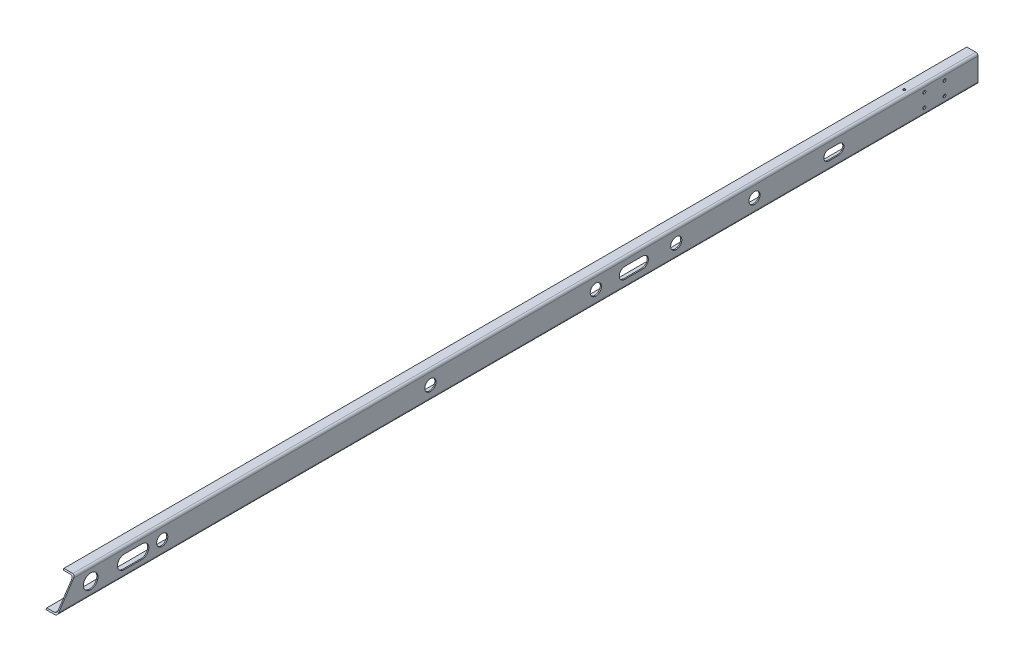
from build123d import *

# Parameters (mm, degrees)
EXTRUDE_1_DEPTH     = 4120
SKETCH_2_R          = 5
CUT_EXTRUDE_1_DEPTH = 10
SKETCH_3_R          = 6.5
SKETCH_3_R_2        = 25
SKETCH_3_R_3        = 22.5
CUT_EXTRUDE_2_DEPTH = 10
CUT_EXTRUDE_3_DEPTH = 10
SKETCH_5_R          = 6.5
CUT_EXTRUDE_4_DEPTH = 10
EXTRUDE_4_DEPTH     = 5
SKETCH_7_R          = 32.5
CUT_EXTRUDE_5_DEPTH = 10
CUT_EXTRUDE_6_DEPTH = 63


with BuildPart() as part:
    # 草图1 → 凸台-拉伸1 (new body)
    with BuildSketch(Plane.XY):
        with BuildLine():
            Line((626.175555556, -48.428888889), (666.175555556, -48.428888889))
            ThreePointArc((666.175555556, -48.428888889), (673.246623367, -45.499956701), (676.175555556, -38.428888889))
            Line((676.175555556, -38.428888889), (676.175555556, 61.571111111))
            ThreePointArc((676.175555556, 61.571111111), (673.246623367, 68.642178923), (666.175555556, 71.571111111))
            Line((666.175555556, 71.571111111), (626.175555556, 71.571111111))
            Line((626.175555556, 71.571111111), (626.175555556, 66.571111111))
            Line((626.175555556, 66.571111111), (661.175555556, 66.571111111))
            ThreePointArc((661.175555556, 66.571111111), (668.246623367, 63.642178923), (671.175555556, 56.571111111))
            Line((671.175555556, 56.571111111), (671.175555556, -33.428888889))
            ThreePointArc((671.175555556, -33.428888889), (668.246623367, -40.499956701), (661.175555556, -43.428888889))
            Line((661.175555556, -43.428888889), (626.175555556, -43.428888889))
            Line((626.175555556, -43.428888889), (626.175555556, -48.428888889))
        make_face()
    extrude(amount=EXTRUDE_1_DEPTH)

    # 草图2 → 切除-拉伸1 (cut)
    with BuildSketch(Plane(origin=(0, 71.571111111, 0), x_dir=(1, 0, 0), z_dir=(0, 1, 0))):
        with Locations(Location((651.175555556, -305, 0), (0, 0, 180))):
            Circle(SKETCH_2_R)
    extrude(amount=-CUT_EXTRUDE_1_DEPTH, mode=Mode.SUBTRACT)

    # 草图3 → 切除-拉伸2 (cut)
    with BuildSketch(Plane(origin=(676.175555556, 0, 0), x_dir=(0, 0, -1), z_dir=(1, 0, 0))):
        with Locations((-225, 41.571111111)):
            Circle(SKETCH_3_R)
        with Locations((-135, 41.571111111)):
            Circle(SKETCH_3_R)
        with Locations((-135, -18.428888889)):
            Circle(SKETCH_3_R)
        with Locations((-225, -18.428888889)):
            Circle(SKETCH_3_R)
        with Locations((-1000, 11.571111111)):
            Circle(SKETCH_3_R_2)
        with Locations((-1350, 11.571111111)):
            Circle(SKETCH_3_R_2)
        with Locations((-3970, 11.571111111)):
            Circle(SKETCH_3_R_3)
        with Locations((-3650, 11.571111111)):
            Circle(SKETCH_3_R_2)
        with Locations((-1710, 11.571111111)):
            Circle(SKETCH_3_R_2)
        with Locations((-2450, 11.571111111)):
            Circle(SKETCH_3_R_2)
        with BuildLine():
            Line((-667.5, 34.071111111), (-622.5, 34.071111111))
            ThreePointArc((-622.5, 34.071111111), (-600, 11.571111111), (-622.5, -10.928888889))
            Line((-622.5, -10.928888889), (-667.5, -10.928888889))
            ThreePointArc((-667.5, -10.928888889), (-690, 11.571111111), (-667.5, 34.071111111))
        make_face()
        with BuildLine():
            Line((-3820, 41.571111111), (-3740, 41.571111111))
            ThreePointArc((-3740, 41.571111111), (-3710, 11.571111111), (-3740, -18.428888889))
            Line((-3740, -18.428888889), (-3820, -18.428888889))
            ThreePointArc((-3820, -18.428888889), (-3850, 11.571111111), (-3820, 41.571111111))
        make_face()
    extrude(amount=-CUT_EXTRUDE_2_DEPTH, mode=Mode.SUBTRACT)

    # 草图4 → 切除-拉伸3 (cut)
    with BuildSketch(Plane(origin=(676.175555556, 0, 0), x_dir=(0, 0, -1), z_dir=(1, 0, 0))):
        with BuildLine():
            Line((-1580, 36.571111111), (-1500, 36.571111111))
            ThreePointArc((-1500, 36.571111111), (-1475, 11.571111111), (-1500, -13.428888889))
            Line((-1500, -13.428888889), (-1580, -13.428888889))
            ThreePointArc((-1580, -13.428888889), (-1605, 11.571111111), (-1580, 36.571111111))
        make_face()
    extrude(amount=-CUT_EXTRUDE_3_DEPTH, mode=Mode.SUBTRACT)

    # 草图5 → 切除-拉伸4 (cut)
    with BuildSketch(Plane(origin=(676.175555556, 0, 0), x_dir=(0, 0, -1), z_dir=(1, 0, 0))):
        with Locations((-150, 41.571111111)):
            Circle(SKETCH_5_R)
        with Locations((-150, -18.428888889)):
            Circle(SKETCH_5_R)
        with Locations((-240, -18.428888889)):
            Circle(SKETCH_5_R)
        with Locations((-240, 41.571111111)):
            Circle(SKETCH_5_R)
    extrude(amount=-CUT_EXTRUDE_4_DEPTH, mode=Mode.SUBTRACT)

    # 草图6 → 凸台-拉伸4 (add)
    with BuildSketch(Plane(origin=(676.175555556, 0, 0), x_dir=(0, 0, -1), z_dir=(1, 0, 0))):
        Polygon((-232.846363418, 52.773090211), (-232.846363418, -32.197108724), (-210.73029119, -32.197108724), (-210.73029119, 54.281769077), align=None)
        Polygon((-141.939510389, 56.005838269), (-142.912723727, -30.568548212), (-122.771795739, -30.568548212), (-119.310073741, -30.568548212), (-119.310073741, 56.005838269), align=None)
    extrude(amount=-EXTRUDE_4_DEPTH)

    # 草图7 → 切除-拉伸5 (cut)
    with BuildSketch(Plane(origin=(676.175555556, 0, 0), x_dir=(0, 0, -1), z_dir=(1, 0, 0))):
        with Locations((-3970, 11.571111111)):
            Circle(SKETCH_7_R)
    extrude(amount=-CUT_EXTRUDE_5_DEPTH, mode=Mode.SUBTRACT)

    # 草图8 → 切除-拉伸6 (cut)
    with BuildSketch(Plane(origin=(676.175555556, 0, 0), x_dir=(0, 0, -1), z_dir=(1, 0, 0))):
        Polygon((-4120, 71.571111111), (-4040, 71.571111111), (-4120, -48.428888889), align=None)
    extrude(amount=-CUT_EXTRUDE_6_DEPTH, mode=Mode.SUBTRACT)


solid = part.part
